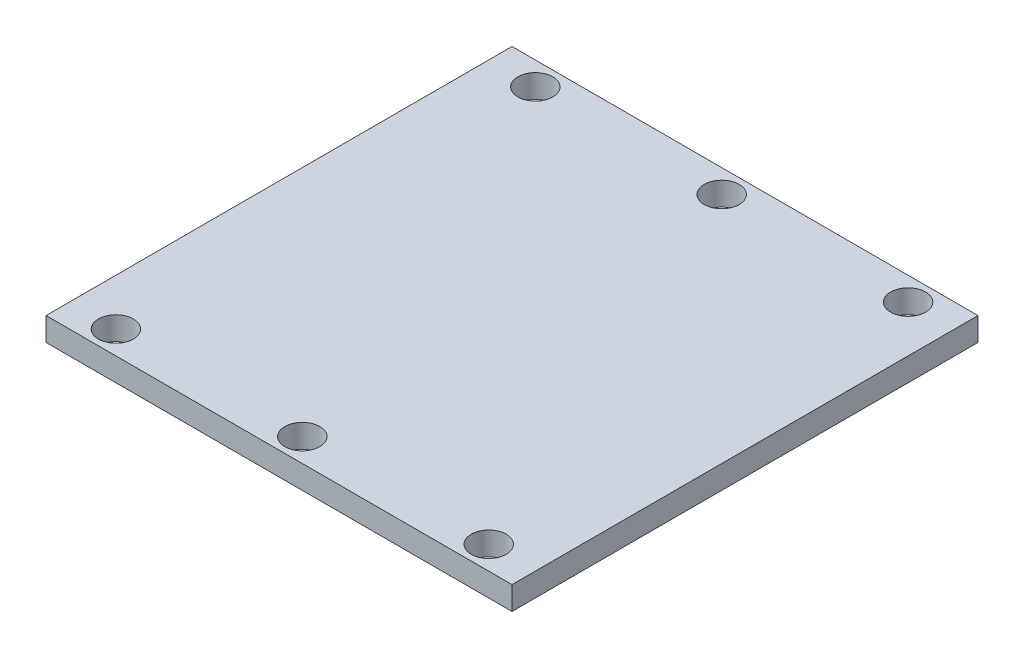
from build123d import *

# Parameters (mm, degrees)
SKETCH1_W            = 200
SKETCH1_H            = 200
BOSS_EXTRUDE1_DEPTH  = 5
SKETCH2_R            = 7.5
CUT_EXTRUDE1_DEPTH   = 10
LPATTERN1_COUNT      = 2
LPATTERN1_PITCH      = 180
LPATTERN1_COUNT_DIR2 = 3
LPATTERN1_PITCH_DIR2 = 80


with BuildPart() as part:
    # Sketch1 → Boss-Extrude1 (new, symmetric)
    with BuildSketch(Plane(origin=(0, 0, 0), x_dir=(1, 0, 0), z_dir=(0, 1, 0))):
        Rectangle(SKETCH1_W, SKETCH1_H)
    extrude(amount=BOSS_EXTRUDE1_DEPTH, both=True)

    # Sketch2 → Cut-Extrude1 (cut)
    with BuildSketch(Plane(origin=(0, 5, 0), x_dir=(1, 0, 0), z_dir=(0, 1, 0))):
        with Locations(Location((80, 90, 0), (0, 0, 270))):
            Circle(SKETCH2_R)
    cut_extrude1 = extrude(amount=-CUT_EXTRUDE1_DEPTH, mode=Mode.SUBTRACT)

    # LPattern1: Cut-Extrude1 2 × 3
    with Locations(*[(-j * LPATTERN1_PITCH_DIR2, 0, i * LPATTERN1_PITCH) for i in range(LPATTERN1_COUNT) for j in range(LPATTERN1_COUNT_DIR2) if (i, j) != (0, 0)]):
        add(cut_extrude1, mode=Mode.SUBTRACT)


solid = part.part
